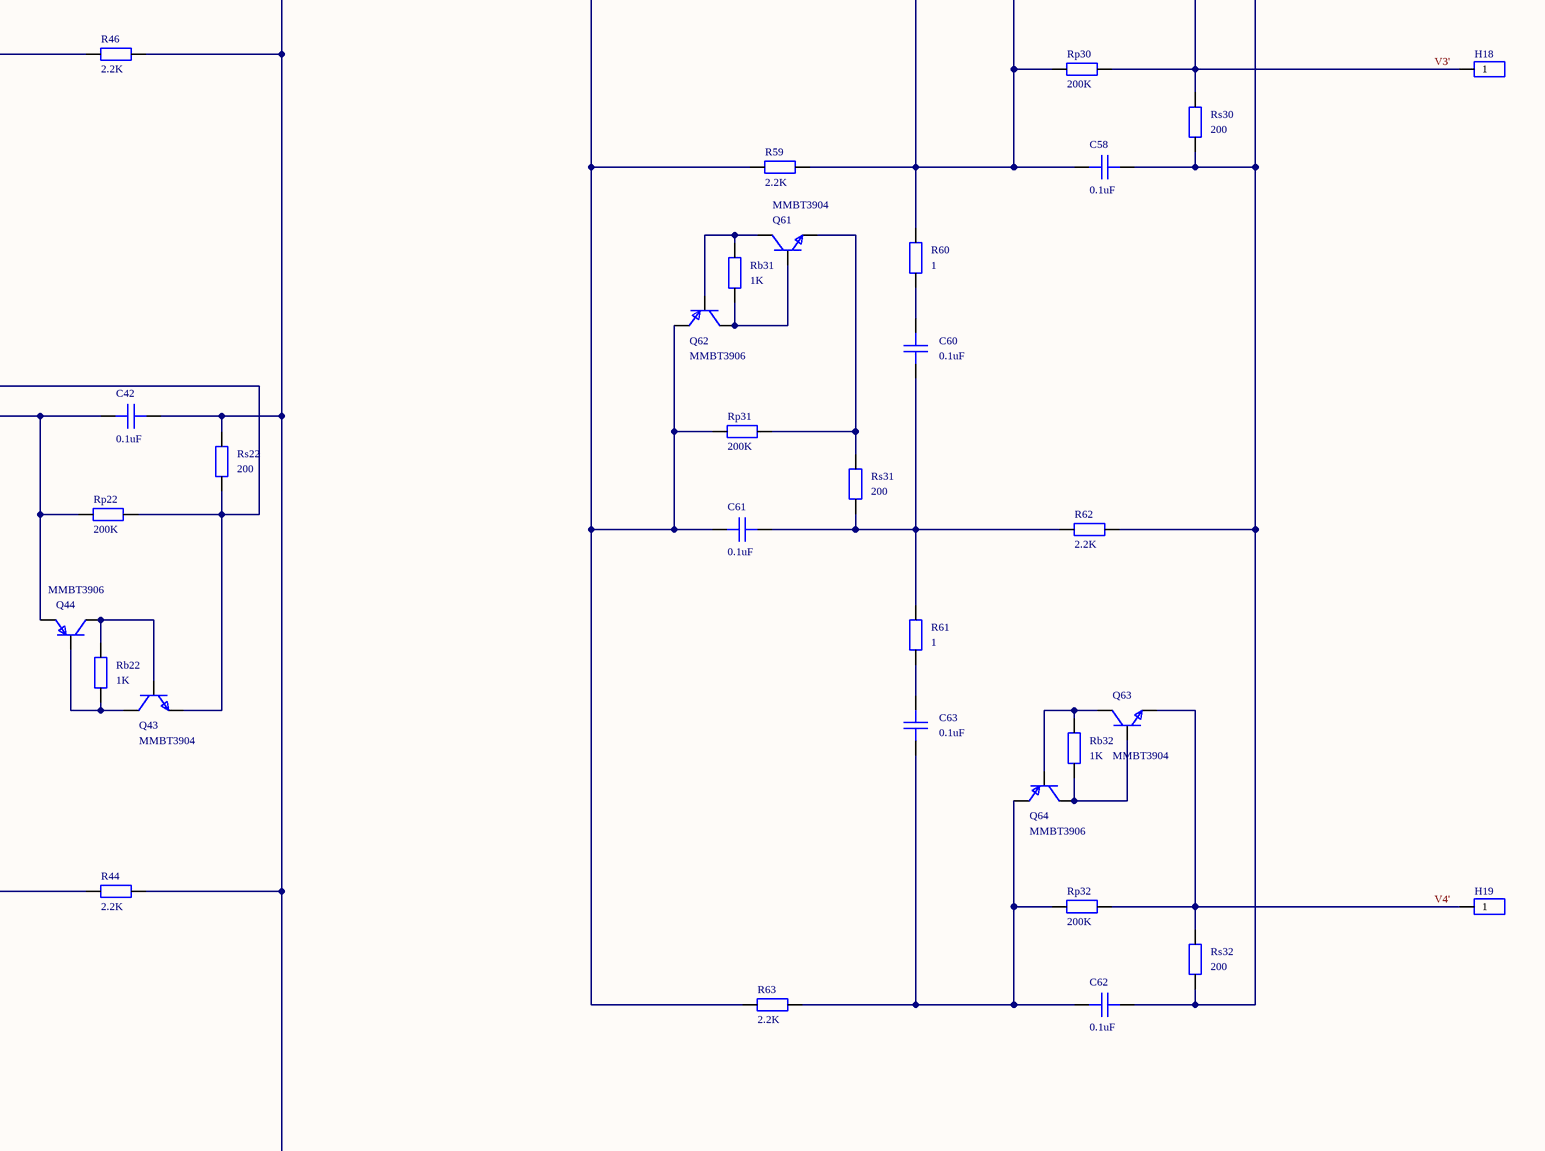
[diagram p0: MISC61260-3.schdoc, bottom right]
# Altium project MISC61260-2.PrjPcb (part 2 of 2)

## Sheet MISC61260-3.schdoc
size 178 x 98 mm; Version: V1.0; @Project Name: MISC61260; @Page Count: 1; @Update Date: 2025-01-10; @Create Date: 2025-01-10; @Schematic Name: MISC61260; @Page No: 1; @Board Name: MISC61260; @Create Time: 21:58:25; @Update Time: 09:22:44

### Parts
C1  0.1uF  [C0402]
C2  0.1uF  [C0402]
C4  0.1uF  [C0402]
C5  0.1uF  [C0402]
C6  0.1uF  [C0402]
C7  0.1uF  [C0402]
C8  0.1uF  [C0402]
C9  0.02uF  [C0402]
C10  0.1uF  [C0402]
C11  0.1uF  [C0402]
C12  0.1uF  [C0402]
C13  0.1uF  [C0402]
C14  0.1uF  [C0402]
C15  0.1uF  [C0402]
C16  0.1uF  [C0402]
C17  0.02uF  [C0402]
C18  0.1uF  [C0402]
C19  0.1uF  [C0402]
C20  0.1uF  [C0402]
C21  0.1uF  [C0402]
C22  0.1uF  [C0402]
C23  0.1uF  [C0402]
C24  0.1uF  [C0402]
C25  0.1uF  [C0402]
C26  0.1uF  [C0402]
C27  0.1uF  [C0402]
C28  0.1uF  [C0402]
C29  0.1uF  [C0402]
C30  0.1uF  [C0402]
C31  0.1uF  [C0402]
C32  0.1uF  [C0402]
C33  0.1uF  [C0402]
C34  0.1uF  [C0402]
C35  0.1uF  [C0402]
C36  0.1uF  [C0402]
C37  0.1uF  [C0402]
C38  0.1uF  [C0402]
C39  0.1uF  [C0402]
C40  0.02uF  [C0402]
C41  0.1uF  [C0402]
C42  0.1uF  [C0402]
C43  0.1uF  [C0402]
C44  0.1uF  [C0402]
C45  0.1uF  [C0402]
C46  0.1uF  [C0402]
C47  0.1uF  [C0402]
C48  0.02uF  [C0402]
C49  0.1uF  [C0402]
C50  0.1uF  [C0402]
C51  0.1uF  [C0402]
C52  0.1uF  [C0402]
C53  0.1uF  [C0402]
C54  0.1uF  [C0402]
C55  0.1uF  [C0402]
C56  0.1uF  [C0402]
C57  0.1uF  [C0402]
C58  0.1uF  [C0402]
C59  0.1uF  [C0402]
C60  0.1uF  [C0402]
C61  0.1uF  [C0402]
C62  0.1uF  [C0402]
C63  0.1uF  [C0402]
H1  (no value)  [HDR-TH_3P-P2.54-V-M]
H2  (no value)  [HDR-TH_1P-V-M_XKB_X4611WV-01I-C28D40]
H3  (no value)  [HDR-TH_1P-V-M_XKB_X4611WV-01I-C28D40]
H4  (no value)  [HDR-TH_1P-V-M_XKB_X4611WV-01I-C28D40]
H5  (no value)  [HDR-TH_1P-V-M_XKB_X4611WV-01I-C28D40]
H6  (no value)  [HDR-TH_1P-V-M_XKB_X4611WV-01I-C28D40]
H7  (no value)  [HDR-TH_1P-V-M_XKB_X4611WV-01I-C28D40]
H9  (no value)  [HDR-TH_1P-V-M_XKB_X4611WV-01I-C28D40]
H10  (no value)  [HDR-TH_1P-V-M_XKB_X4611WV-01I-C28D40]
H12  (no value)  [HDR-TH_1P-V-M_XKB_X4611WV-01I-C28D40]
H13  (no value)  [HDR-TH_1P-V-M_XKB_X4611WV-01I-C28D40]
H14  (no value)  [HDR-TH_1P-V-M_XKB_X4611WV-01I-C28D40]
H15  (no value)  [HDR-TH_1P-V-M_XKB_X4611WV-01I-C28D40]
H16  (no value)  [HDR-TH_1P-V-M_XKB_X4611WV-01I-C28D40]
H17  (no value)  [HDR-TH_1P-V-M_XKB_X4611WV-01I-C28D40]
H18  (no value)  [HDR-TH_1P-V-M_XKB_X4611WV-01I-C28D40]
H19  (no value)  [HDR-TH_1P-V-M_XKB_X4611WV-01I-C28D40]
H20  (no value)  [HDR-TH_1P-V-M_XKB_X4611WV-01I-C28D40]
H21  (no value)  [HDR-TH_3P-P2.54-V-M]
H22  (no value)  [HDR-TH_1P-V-M_XKB_X4611WV-01I-C28D40]
Q1  MMBT3906  [SOT-23-3_L2.9-W1.3-P1.90-LS2.4-BR]
Q2  MMBT3904  [SOT-23-3_L2.9-W1.3-P1.90-LS2.4-BR]
Q3  MMBT3906  [SOT-23-3_L2.9-W1.3-P1.90-LS2.4-BR]
Q4  MMBT3904  [SOT-23-3_L2.9-W1.3-P1.90-LS2.4-BR]
Q5  MMBT3904  [SOT-23-3_L2.9-W1.3-P1.90-LS2.4-BR]
Q6  MMBT3906  [SOT-23-3_L2.9-W1.3-P1.90-LS2.4-BR]
Q7  MMBT3904  [SOT-23-3_L2.9-W1.3-P1.90-LS2.4-BR]
Q8  MMBT3906  [SOT-23-3_L2.9-W1.3-P1.90-LS2.4-BR]
Q9  MMBT3904  [SOT-23-3_L2.9-W1.3-P1.90-LS2.4-BR]
Q10  MMBT3906  [SOT-23-3_L2.9-W1.3-P1.90-LS2.4-BR]
Q11  MMBT3904  [SOT-23-3_L2.9-W1.3-P1.90-LS2.4-BR]
Q12  MMBT3906  [SOT-23-3_L2.9-W1.3-P1.90-LS2.4-BR]
Q13  MMBT3904  [SOT-23-3_L2.9-W1.3-P1.90-LS2.4-BR]
Q14  MMBT3906  [SOT-23-3_L2.9-W1.3-P1.90-LS2.4-BR]
Q15  MMBT3904  [SOT-23-3_L2.9-W1.3-P1.90-LS2.4-BR]
Q16  MMBT3906  [SOT-23-3_L2.9-W1.3-P1.90-LS2.4-BR]
Q17  MMBT3904  [SOT-23-3_L2.9-W1.3-P1.90-LS2.4-BR]
Q18  MMBT3906  [SOT-23-3_L2.9-W1.3-P1.90-LS2.4-BR]
Q19  MMBT3904  [SOT-23-3_L2.9-W1.3-P1.90-LS2.4-BR]
Q20  MMBT3906  [SOT-23-3_L2.9-W1.3-P1.90-LS2.4-BR]
Q21  MMBT3904  [SOT-23-3_L2.9-W1.3-P1.90-LS2.4-BR]
Q22  MMBT3906  [SOT-23-3_L2.9-W1.3-P1.90-LS2.4-BR]
Q23  MMBT3904  [SOT-23-3_L2.9-W1.3-P1.90-LS2.4-BR]
Q24  MMBT3906  [SOT-23-3_L2.9-W1.3-P1.90-LS2.4-BR]
Q25  MMBT3904  [SOT-23-3_L2.9-W1.3-P1.90-LS2.4-BR]
Q26  MMBT3906  [SOT-23-3_L2.9-W1.3-P1.90-LS2.4-BR]
Q27  MMBT3904  [SOT-23-3_L2.9-W1.3-P1.90-LS2.4-BR]
Q28  MMBT3906  [SOT-23-3_L2.9-W1.3-P1.90-LS2.4-BR]
Q29  MMBT3904  [SOT-23-3_L2.9-W1.3-P1.90-LS2.4-BR]
Q30  MMBT3906  [SOT-23-3_L2.9-W1.3-P1.90-LS2.4-BR]
Q31  MMBT3904  [SOT-23-3_L2.9-W1.3-P1.90-LS2.4-BR]
Q32  MMBT3906  [SOT-23-3_L2.9-W1.3-P1.90-LS2.4-BR]
Q33  MMBT3904  [SOT-23-3_L2.9-W1.3-P1.90-LS2.4-BR]
Q34  MMBT3906  [SOT-23-3_L2.9-W1.3-P1.90-LS2.4-BR]
Q35  MMBT3904  [SOT-23-3_L2.9-W1.3-P1.90-LS2.4-BR]
Q36  MMBT3906  [SOT-23-3_L2.9-W1.3-P1.90-LS2.4-BR]
Q37  MMBT3904  [SOT-23-3_L2.9-W1.3-P1.90-LS2.4-BR]
Q38  MMBT3906  [SOT-23-3_L2.9-W1.3-P1.90-LS2.4-BR]
Q39  MMBT3904  [SOT-23-3_L2.9-W1.3-P1.90-LS2.4-BR]
Q40  MMBT3906  [SOT-23-3_L2.9-W1.3-P1.90-LS2.4-BR]
Q41  MMBT3904  [SOT-23-3_L2.9-W1.3-P1.90-LS2.4-BR]
Q42  MMBT3906  [SOT-23-3_L2.9-W1.3-P1.90-LS2.4-BR]
Q43  MMBT3904  [SOT-23-3_L2.9-W1.3-P1.90-LS2.4-BR]
Q44  MMBT3906  [SOT-23-3_L2.9-W1.3-P1.90-LS2.4-BR]
Q45  MMBT3904  [SOT-23-3_L2.9-W1.3-P1.90-LS2.4-BR]
Q46  MMBT3906  [SOT-23-3_L2.9-W1.3-P1.90-LS2.4-BR]
Q47  MMBT3904  [SOT-23-3_L2.9-W1.3-P1.90-LS2.4-BR]
Q48  MMBT3906  [SOT-23-3_L2.9-W1.3-P1.90-LS2.4-BR]
Q49  MMBT3904  [SOT-23-3_L2.9-W1.3-P1.90-LS2.4-BR]
Q50  MMBT3906  [SOT-23-3_L2.9-W1.3-P1.90-LS2.4-BR]
Q51  MMBT3904  [SOT-23-3_L2.9-W1.3-P1.90-LS2.4-BR]
Q52  MMBT3906  [SOT-23-3_L2.9-W1.3-P1.90-LS2.4-BR]
Q53  MMBT3904  [SOT-23-3_L2.9-W1.3-P1.90-LS2.4-BR]
Q54  MMBT3906  [SOT-23-3_L2.9-W1.3-P1.90-LS2.4-BR]
Q55  MMBT3904  [SOT-23-3_L2.9-W1.3-P1.90-LS2.4-BR]
Q56  MMBT3906  [SOT-23-3_L2.9-W1.3-P1.90-LS2.4-BR]
Q57  MMBT3904  [SOT-23-3_L2.9-W1.3-P1.90-LS2.4-BR]
Q58  MMBT3906  [SOT-23-3_L2.9-W1.3-P1.90-LS2.4-BR]
Q59  MMBT3904  [SOT-23-3_L2.9-W1.3-P1.90-LS2.4-BR]
Q60  MMBT3906  [SOT-23-3_L2.9-W1.3-P1.90-LS2.4-BR]
Q61  MMBT3904  [SOT-23-3_L2.9-W1.3-P1.90-LS2.4-BR]
Q62  MMBT3906  [SOT-23-3_L2.9-W1.3-P1.90-LS2.4-BR]
Q63  MMBT3904  [SOT-23-3_L2.9-W1.3-P1.90-LS2.4-BR]
Q64  MMBT3906  [SOT-23-3_L2.9-W1.3-P1.90-LS2.4-BR]
R1  1  [R0402]
R3  2.2K  [R0402]
R4  2.2K  [R0402]
R5  1  [R0402]
R6  1  [R0402]
R7  2.2K  [R0402]
R9  2.2K  [R0402]
R10  1  [R0402]
R11  1  [R0402]
R12  1  [R0402]
R13  2.2K  [R0402]
R14  2.2K  [R0402]
R15  1  [R0402]
R16  2.2K  [R0402]
R17  2.2K  [R0402]
R18  1  [R0402]
R19  1  [R0402]
R20  2.2K  [R0402]
R21  2.55K  [R0402]
R22  1  [R0402]
R23  1  [R0402]
R24  2.2K  [R0402]
R25  2.2K  [R0402]
R26  1  [R0402]
R27  1  [R0402]
R28  2.2K  [R0402]
R29  2.2K  [R0402]
R30  1  [R0402]
R31  1  [R0402]
R32  2.2K  [R0402]
R33  1  [R0402]
R34  1  [R0402]
R35  2.2K  [R0402]
R36  2.2K  [R0402]
R37  1  [R0402]
R38  2.2K  [R0402]
R39  2.2K  [R0402]
R40  1  [R0402]
R41  1  [R0402]
R42  1  [R0402]
R43  2.2K  [R0402]
R44  2.2K  [R0402]
R45  1  [R0402]
R46  2.2K  [R0402]
R47  2.2K  [R0402]
R48  1  [R0402]
R49  1  [R0402]
R50  2.2K  [R0402]
R51  2.55K  [R0402]
R52  1  [R0402]
R53  1  [R0402]
R54  2.2K  [R0402]
R55  2.2K  [R0402]
R56  1  [R0402]
R57  1  [R0402]
R58  2.2K  [R0402]
R59  2.2K  [R0402]
R60  1  [R0402]
R61  1  [R0402]
R62  2.2K  [R0402]
R63  2.2K  [R0402]
Rb1  1K  [R0402]
Rb2  1K  [R0402]
Rb3  1K  [R0402]
Rb4  1K  [R0402]
Rb5  1K  [R0402]
Rb6  1K  [R0402]
Rb7  1K  [R0402]
Rb8  1K  [R0402]
Rb9  1K  [R0402]
Rb10  1K  [R0402]
Rb11  1K  [R0402]
Rb12  1K  [R0402]
Rb13  1K  [R0402]
Rb14  1K  [R0402]
Rb15  1K  [R0402]
Rb16  1K  [R0402]
Rb17  1K  [R0402]
Rb18  1K  [R0402]
Rb19  1K  [R0402]
Rb20  1K  [R0402]
Rb21  1K  [R0402]
Rb22  1K  [R0402]
Rb23  1K  [R0402]
Rb24  1K  [R0402]
Rb25  1K  [R0402]
Rb26  1K  [R0402]
Rb27  1K  [R0402]
Rb28  1K  [R0402]
Rb29  1K  [R0402]
Rb30  1K  [R0402]
Rb31  1K  [R0402]
Rb32  1K  [R0402]
Rp1  200K  [R0402]
Rp2  200K  [R0402]
Rp3  200K  [R0402]
Rp4  200K  [R0402]
Rp5  200K  [R0402]
Rp6  200K  [R0402]
Rp7  200K  [R0402]
Rp8  200K  [R0402]
Rp9  200K  [R0402]
Rp10  200K  [R0402]
Rp11  200K  [R0402]
Rp12  200K  [R0402]
Rp13  200K  [R0402]
Rp14  200K  [R0402]
Rp15  200K  [R0402]
Rp16  200K  [R0402]
Rp17  200K  [R0402]
Rp18  200K  [R0402]
Rp19  200K  [R0402]
Rp20  200K  [R0402]
Rp21  200K  [R0402]
Rp22  200K  [R0402]
Rp23  200K  [R0402]
Rp24  200K  [R0402]
Rp25  200K  [R0402]
Rp26  200K  [R0402]
Rp27  200K  [R0402]
Rp28  200K  [R0402]
Rp29  200K  [R0402]
Rp30  200K  [R0402]
Rp31  200K  [R0402]
Rp32  200K  [R0402]
Rs1  200  [R0402]
Rs2  200  [R0402]
Rs3  200  [R0402]
Rs4  200  [R0402]
Rs5  200  [R0402]
Rs6  200  [R0402]
Rs7  200  [R0402]
Rs8  200  [R0402]
Rs9  200  [R0402]
Rs10  200  [R0402]
Rs11  200  [R0402]
Rs12  200  [R0402]
Rs13  200  [R0402]
Rs14  200  [R0402]
Rs15  200  [R0402]
Rs16  200  [R0402]
Rs17  200  [R0402]
Rs18  200  [R0402]
Rs19  200  [R0402]
Rs20  200  [R0402]
Rs21  200  [R0402]
Rs22  200  [R0402]
Rs23  200  [R0402]
Rs24  200  [R0402]
Rs25  200  [R0402]
Rs26  200  [R0402]
Rs27  200  [R0402]
Rs28  200  [R0402]
Rs29  200  [R0402]
Rs30  200  [R0402]
Rs31  200  [R0402]
Rs32  200  [R0402]

### Nets
B1: C4.2 H1.2 R1.2 R3.1 Rs1.2
B1': C10.2 H21.2 R11.2 R14.1 Rs5.2
B2: C33.2 H20.1 R33.2 R36.1 Rs17.2
B2': C41.2 H22.1 R41.2 R44.1 Rs21.2
GND: C5.2 C7.2 C11.2 C15.2 C19.2 C23.2 C27.2 C31.2 C34.2 C38.2 C42.2 C46.2 C50.2 C54.2 C58.2 C62.2 H1.3 H21.3 R3.2 R7.2 R14.2 R16.2 R21.2 R24.2 R28.2 R32.2 R36.2 R38.2 R44.2 R46.2 R51.2 R54.2 R58.2 R62.2 Rs2.2 Rs4.2 Rs6.2 Rs8.2 Rs10.2 Rs12.2 Rs14.2 Rs16.2 Rs18.2 Rs20.2 Rs22.2 Rs24.2 Rs26.2 Rs28.2 Rs30.2 Rs32.2
V1: H6.1 Q19.2(E) Rp10.2 Rs10.1
V1': H16.1 Q51.2(E) Rp26.2 Rs26.1
V2: H7.1 Q23.2(E) Rp12.2 Rs12.1
V2': H17.1 Q55.2(E) Rp28.2 Rs28.1
V3: H9.1 Q27.2(E) Rp14.2 Rs14.1
V3': H18.1 Q59.2(E) Rp30.2 Rs30.1
V4: H10.1 Q31.2(E) Rp16.2 Rs16.1
V4': H19.1 Q63.2(E) Rp32.2 Rs32.1
V+: C4.1 C6.1 C10.1 C14.1 C18.1 C22.1 C26.1 C30.1 C31.1 C32.1 C33.1 C37.1 C41.1 C45.1 C49.1 C53.1 C57.1 C61.1 H1.1 H21.1 Q3.2(E) Q6.2(E) Q10.2(E) Q14.2(E) Q18.2(E) Q22.2(E) Q26.2(E) Q30.2(E) Q32.2(E) Q34.2(E) Q38.2(E) Q42.2(E) Q46.2(E) Q50.2(E) Q54.2(E) Q58.2(E) Q62.2(E) R4.1 R9.1 R13.1 R17.1 R20.1 R25.1 R29.1 R35.1 R39.1 R43.1 R47.1 R50.1 R55.1 R59.1 R63.1 Rp1.1 Rp3.1 Rp5.1 Rp7.1 Rp9.1 Rp11.1 Rp13.1 Rp15.1 Rp16.1 Rp17.1 Rp19.1 Rp21.1 Rp23.1 Rp25.1 Rp27.1 Rp29.1 Rp31.1  [also labelled V+']
VL1: H2.1 Q4.2(E) Rp2.2 Rs2.1
VL1': H12.1 Q35.2(E) Rp18.2 Rs18.1
VL2: H3.1 Q7.2(E) Rp4.2 Rs4.1
VL2': H13.1 Q39.2(E) Rp20.2 Rs20.1
VR1: H5.1 Q11.2(E) Rp6.2 Rs6.1
VR1': H15.1 Q43.2(E) Rp22.2 Rs22.1
VR2: H4.1 Q15.2(E) Rp8.2 Rs8.1
VR2': H14.1 Q47.2(E) Rp24.2 Rs24.1
NetC1_1: C1.1 C6.2 R6.2 R7.1 Rs3.2
NetC1_2: C1.2 R5.1
NetC2_1: C2.1 C5.1 Q1.2(E) R4.2 R5.2 Rp2.1
NetC2_2: C2.2 R1.1
NetC7_1: C7.1 C8.1 Q8.2(E) R9.2 R10.2 Rp4.1
NetC8_2: C8.2 R6.1
NetC9_1: C9.1 C17.1 C18.2 R19.2 R21.1 Rs9.2
NetC9_2: C9.2 R10.1
NetC11_1: C11.1 C12.1 Q12.2(E) R12.2 R13.2 Rp6.1
NetC12_2: C12.2 R11.1
NetC13_1: C13.1 C14.2 R15.2 R16.1 Rs7.2
NetC13_2: C13.2 R12.1
NetC15_1: C15.1 C16.1 Q16.2(E) R17.2 R18.2 Rp8.1
NetC16_2: C16.2 R15.1
NetC17_2: C17.2 R18.1
NetC19_1: C19.1 C20.1 Q20.2(E) R20.2 R22.2 Rp10.1
NetC20_2: C20.2 R19.1
NetC21_1: C21.1 C22.2 R23.2 R24.1 Rs11.2
NetC21_2: C21.2 R22.1
NetC23_1: C23.1 C24.1 Q24.2(E) R25.2 R26.2 Rp12.1
NetC24_2: C24.2 R23.1
NetC25_1: C25.1 C26.2 R27.2 R28.1 Rs13.2
NetC25_2: C25.2 R26.1
NetC27_1: C27.1 C28.1 Q28.2(E) R29.2 R30.2 Rp14.1
NetC28_2: C28.2 R27.1
NetC29_1: C29.1 C30.2 R31.2 R32.1 Rs15.2
NetC29_2: C29.2 R30.1
NetC32_2: C32.2 R31.1
NetC34_1: C34.1 C35.1 Q36.2(E) R34.2 R35.2 Rp18.1
NetC35_2: C35.2 R33.1
NetC36_1: C36.1 C37.2 R37.2 R38.1 Rs19.2
NetC36_2: C36.2 R34.1
NetC38_1: C38.1 C39.1 Q40.2(E) R39.2 R40.2 Rp20.1
NetC39_2: C39.2 R37.1
NetC40_1: C40.1 C48.1 C49.2 R49.2 R51.1 Rs25.2
NetC40_2: C40.2 R40.1
NetC42_1: C42.1 C43.1 Q44.2(E) R42.2 R43.2 Rp22.1
NetC43_2: C43.2 R41.1
NetC44_1: C44.1 C45.2 R45.2 R46.1 Rs23.2
NetC44_2: C44.2 R42.1
NetC46_1: C46.1 C47.1 Q48.2(E) R47.2 R48.2 Rp24.1
NetC47_2: C47.2 R45.1
NetC48_2: C48.2 R48.1
NetC50_1: C50.1 C51.1 Q52.2(E) R50.2 R52.2 Rp26.1
NetC51_2: C51.2 R49.1
NetC52_1: C52.1 C53.2 R53.2 R54.1 Rs27.2
NetC52_2: C52.2 R52.1
NetC54_1: C54.1 C55.1 Q56.2(E) R55.2 R56.2 Rp28.1
NetC55_2: C55.2 R53.1
NetC56_1: C56.1 C57.2 R57.2 R58.1 Rs29.2
NetC56_2: C56.2 R56.1
NetC58_1: C58.1 C59.1 Q60.2(E) R59.2 R60.2 Rp30.1
NetC59_2: C59.2 R57.1
NetC60_1: C60.1 C61.2 R61.2 R62.1 Rs31.2
NetC60_2: C60.2 R60.1
NetC62_1: C62.1 C63.1 Q64.2(E) R63.2 Rp32.1
NetC63_2: C63.2 R61.1
NetQ1_1: Q1.1(B) Q4.3(C) Rb2.2
NetQ1_3: Q1.3(C) Q4.1(B) Rb2.1
NetQ2_1: Q2.1(B) Q3.3(C) Rb1.1
NetQ2_2: Q2.2(E) Rp1.2 Rs1.1
NetQ2_3: Q2.3(C) Q3.1(B) Rb1.2
NetQ5_1: Q5.1(B) Q6.3(C) Rb3.1
NetQ5_2: Q5.2(E) Rp3.2 Rs3.1
NetQ5_3: Q5.3(C) Q6.1(B) Rb3.2
NetQ7_1: Q7.1(B) Q8.3(C) Rb4.1
NetQ7_3: Q7.3(C) Q8.1(B) Rb4.2
NetQ9_1: Q9.1(B) Q10.3(C) Rb5.1
NetQ9_2: Q9.2(E) Rp5.2 Rs5.1
NetQ9_3: Q9.3(C) Q10.1(B) Rb5.2
NetQ11_1: Q11.1(B) Q12.3(C) Rb6.1
NetQ11_3: Q11.3(C) Q12.1(B) Rb6.2
NetQ13_1: Q13.1(B) Q14.3(C) Rb7.1
NetQ13_2: Q13.2(E) Rp7.2 Rs7.1
NetQ13_3: Q13.3(C) Q14.1(B) Rb7.2
NetQ15_1: Q15.1(B) Q16.3(C) Rb8.1
NetQ15_3: Q15.3(C) Q16.1(B) Rb8.2
NetQ17_1: Q17.1(B) Q18.3(C) Rb9.1
NetQ17_2: Q17.2(E) Rp9.2 Rs9.1
NetQ17_3: Q17.3(C) Q18.1(B) Rb9.2
NetQ19_1: Q19.1(B) Q20.3(C) Rb10.1
NetQ19_3: Q19.3(C) Q20.1(B) Rb10.2
NetQ21_1: Q21.1(B) Q22.3(C) Rb11.1
NetQ21_2: Q21.2(E) Rp11.2 Rs11.1
NetQ21_3: Q21.3(C) Q22.1(B) Rb11.2
NetQ23_1: Q23.1(B) Q24.3(C) Rb12.1
NetQ23_3: Q23.3(C) Q24.1(B) Rb12.2
NetQ25_1: Q25.1(B) Q26.3(C) Rb13.1
NetQ25_2: Q25.2(E) Rp13.2 Rs13.1
NetQ25_3: Q25.3(C) Q26.1(B) Rb13.2
NetQ27_1: Q27.1(B) Q28.3(C) Rb14.1
NetQ27_3: Q27.3(C) Q28.1(B) Rb14.2
NetQ29_1: Q29.1(B) Q30.3(C) Rb15.1
NetQ29_2: Q29.2(E) Rp15.2 Rs15.1
NetQ29_3: Q29.3(C) Q30.1(B) Rb15.2
NetQ31_1: Q31.1(B) Q32.3(C) Rb16.1
NetQ31_3: Q31.3(C) Q32.1(B) Rb16.2
NetQ33_1: Q33.1(B) Q34.3(C) Rb17.1
NetQ33_2: Q33.2(E) Rp17.2 Rs17.1
NetQ33_3: Q33.3(C) Q34.1(B) Rb17.2
NetQ35_1: Q35.1(B) Q36.3(C) Rb18.1
NetQ35_3: Q35.3(C) Q36.1(B) Rb18.2
NetQ37_1: Q37.1(B) Q38.3(C) Rb19.1
NetQ37_2: Q37.2(E) Rp19.2 Rs19.1
NetQ37_3: Q37.3(C) Q38.1(B) Rb19.2
NetQ39_1: Q39.1(B) Q40.3(C) Rb20.1
NetQ39_3: Q39.3(C) Q40.1(B) Rb20.2
NetQ41_1: Q41.1(B) Q42.3(C) Rb21.1
NetQ41_2: Q41.2(E) Rp21.2 Rs21.1
NetQ41_3: Q41.3(C) Q42.1(B) Rb21.2
NetQ43_1: Q43.1(B) Q44.3(C) Rb22.1
NetQ43_3: Q43.3(C) Q44.1(B) Rb22.2
NetQ45_1: Q45.1(B) Q46.3(C) Rb23.1
NetQ45_2: Q45.2(E) Rp23.2 Rs23.1
NetQ45_3: Q45.3(C) Q46.1(B) Rb23.2
NetQ47_1: Q47.1(B) Q48.3(C) Rb24.1
NetQ47_3: Q47.3(C) Q48.1(B) Rb24.2
NetQ49_1: Q49.1(B) Q50.3(C) Rb25.1
NetQ49_2: Q49.2(E) Rp25.2 Rs25.1
NetQ49_3: Q49.3(C) Q50.1(B) Rb25.2
NetQ51_1: Q51.1(B) Q52.3(C) Rb26.1
NetQ51_3: Q51.3(C) Q52.1(B) Rb26.2
NetQ53_1: Q53.1(B) Q54.3(C) Rb27.1
NetQ53_2: Q53.2(E) Rp27.2 Rs27.1
NetQ53_3: Q53.3(C) Q54.1(B) Rb27.2
NetQ55_1: Q55.1(B) Q56.3(C) Rb28.1
NetQ55_3: Q55.3(C) Q56.1(B) Rb28.2
NetQ57_1: Q57.1(B) Q58.3(C) Rb29.1
NetQ57_2: Q57.2(E) Rp29.2 Rs29.1
NetQ57_3: Q57.3(C) Q58.1(B) Rb29.2
NetQ59_1: Q59.1(B) Q60.3(C) Rb30.1
NetQ59_3: Q59.3(C) Q60.1(B) Rb30.2
NetQ61_1: Q61.1(B) Q62.3(C) Rb31.1
NetQ61_2: Q61.2(E) Rp31.2 Rs31.1
NetQ61_3: Q61.3(C) Q62.1(B) Rb31.2
NetQ63_1: Q63.1(B) Q64.3(C) Rb32.1
NetQ63_3: Q63.3(C) Q64.1(B) Rb32.2

### Notes on the sheet
- 2025-01-10
- Schematic
- Sheet
- Part code
- P1
- Checked
- Drawn
- Revision
- Size
- page
- Total
- A4
- 1

### Library data of the parts
C1 C2 C4-C63 = CAP_0402: ConvertToPcb: yes; SymbolName: CapAcitance; ModelId: 36a51122f27c49738f86b3bfa98863e0; ModelName: C0402_L1.0-W0.5-H0.5; ModelTransform: 39.37,19.685,0,0,0,0,0,0,0; Device: CAP_0402; AddInBom: yes; Supplier Footprint: 0402; FootprintName: C0402
  C1 C2 C4-C8 C10-C16 C18-C39 C41-C47 C49-C63: Value: 0.1uF
  C9 C17 C40 C48: Value: 0.02uF
H1 H21 = HDR-M_2.54_1x3P: Symbol: PZ254V-11-03P_C2937625; ConvertToPcb: yes; ModelId: bb473b6d38ff42a99216a4fcdbdcc4cb; ModelName: HDR-TH_3P-P2.54-M-LI-1X3P; ModelTransform: 299.9994,100,0,0,0,0,0,0,-118.11; Device: HDR-M_2.54_1x3P; AddInBom: yes; SupplierPart: C2937625; Supplier Footprint: 插件; FootprintName: HDR-TH_3P-P2.54-V-M
H2-H7 H9 H10 H12-H20 H22 = HDR-M_2.54_1x1P: Symbol: HDR_1x1; ConvertToPcb: yes; ModelId: 95857080d3cc4057a19a22ccce05e171; ModelTransform: 78.74,79.1337,0,0,0,0,0,0,-110.236; Device: HDR-M_2.54_1x1P; AddInBom: yes; SupplierPart: C81276; Supplier Footprint: 插件; FootprintName: HDR-TH_1P-V-M_XKB_X4611WV-01I-C28D40; JLCPCB Part Class: Extended Part; ModelName: HDR-TH_1P-V-M_XKB_X4611WV-01I-C28D40
Q1 Q3 Q6 Q8 Q10 Q12 Q14 Q16 Q18 Q20 Q22 Q24 Q26 Q28 Q30 Q32 Q34 Q36 Q38 Q40 Q42 Q44 Q46 Q48 Q50 Q52 Q54 Q56 Q58 Q60 Q62 Q64 = MMBT3906-13-01-F: transistor type: -; collector current (Ic): -; collector-emitter breakdown voltage (Vceo): -; power (Pd): -;; Manufacturer: DIODES(美台); AddInBom: yes; ModelId: c62791f0466c4ae2a892c056b845b0ca; ModelName: SOT-23-3P_L2.9-W1.3-H1.0-LS2.4-P0.95; ModelTransform: 98.425,114.173,0,180,0,0,0.0005,-0.0005,0; Symbol: MMBT3906-13-01-F; Manufacturer Part: MMBT3906; Device: MMBT3906-13-01-F; LCSC Part Name: MMBT3906-13-01-F; SupplierPart: C526675; Supplier Footprint: SOT-23-3; JLCPCB Part Class: Extended library; Supplier: LCSC; ConvertToPcb: yes; FootprintName: SOT-23-3_L2.9-W1.3-P1.90-LS2.4-BR; Transistor Type: -; Collector Current (Ic): -; Collector-Emitter Breakdown Voltage (Vceo): -; Power Dissipation (Pd): -; Transition Frequency (fT): -; Collector Cut-Off Current (Icbo): -; Collector-Emitter Saturation Voltage (VCE(sat)@Ic,Ib): -
Q2 Q4 Q5 Q7 Q9 Q11 Q13 Q15 Q17 Q19 Q21 Q23 Q25 Q27 Q29 Q31 Q33 Q35 Q37 Q39 Q41 Q43 Q45 Q47 Q49 Q51 Q53 Q55 Q57 Q59 Q61 Q63 = MMBT3904(RANGE:100-300): transistor type: NPN; collector current (Ic): 200mA; collector-emitter breakdown voltage (Vceo): 40V; power (Pd): 200mW; DC current gain (hFE@Ic,Vce): 100@10mA,1V;; Manufacturer: CJ(江苏长电/长晶); AddInBom: yes; ModelId: c62791f0466c4ae2a892c056b845b0ca; ModelName: SOT-23-3P_L2.9-W1.3-H1.0-LS2.4-P0.95; ModelTransform: 98.425,114.173,0,180,0,0,0.0005,-0.0005,0; Transition Frequency (fT): 300MHz; Collector Cut-Off Current (Icbo): 100nA; Collector-Emitter Saturation Voltage (VCE(sat)@Ic,Ib): 300mV@50mA,5mA; Symbol: MMBT3904; Manufacturer Part: MMBT3904; Device: MMBT3904(RANGE:100-300); LCSC Part Name: NPN 电流:200mA 耐压:40V hfe=100~300; SupplierPart: C20526; Supplier Footprint: SOT-23; Datasheet: example.com/20220704/70F575FB75061E03F919270A6BB8BA7F.pdf; Supplier: LCSC; ConvertToPcb: yes; FootprintName: SOT-23-3_L2.9-W1.3-P1.90-LS2.4-BR; Transistor Type: NPN; Collector Current (Ic): 200mA; Collector-Emitter Breakdown Voltage (Vceo): 40V; Power Dissipation (Pd): 200mW; DC Current Gain (hFE@Ic,Vce): 100@10mA,1V; Operating Temperature: -
R1 R3-R7 R9-R63 Rb1-Rb32 Rp1-Rp32 Rs1-Rs32 = Res_0402: Symbol: Resistor; ConvertToPcb: yes; ModelId: 671aefced39d4c318694bba8bd8efd39; ModelName: R0402_L1.0-W0.5-H0.5; ModelTransform: 39.37,19.685,0,0,0,0,0,0.0005,0; Device: Res_0402; AddInBom: yes; Supplier Footprint: 0402; FootprintName: R0402
  R1 R5 R6 R10-R12 R15 R18 R19 R22 R23 R26 R27 R30 R31 R33 R34 R37 R40-R42 R45 R48 R49 R52 R53 R56 R57 R60 R61: Value: 1
  R3 R4 R7 R9 R13 R14 R16 R17 R20 R24 R25 R28 R29 R32 R35 R36 R38 R39 R43 R44 R46 R47 R50 R54 R55 R58 R59 R62 R63: Value: 2.2K
  R21 R51: Value: 2.55K
  Rb1-Rb32: Value: 1K
  Rp1-Rp32: Value: 200K
  Rs1-Rs32: Value: 200